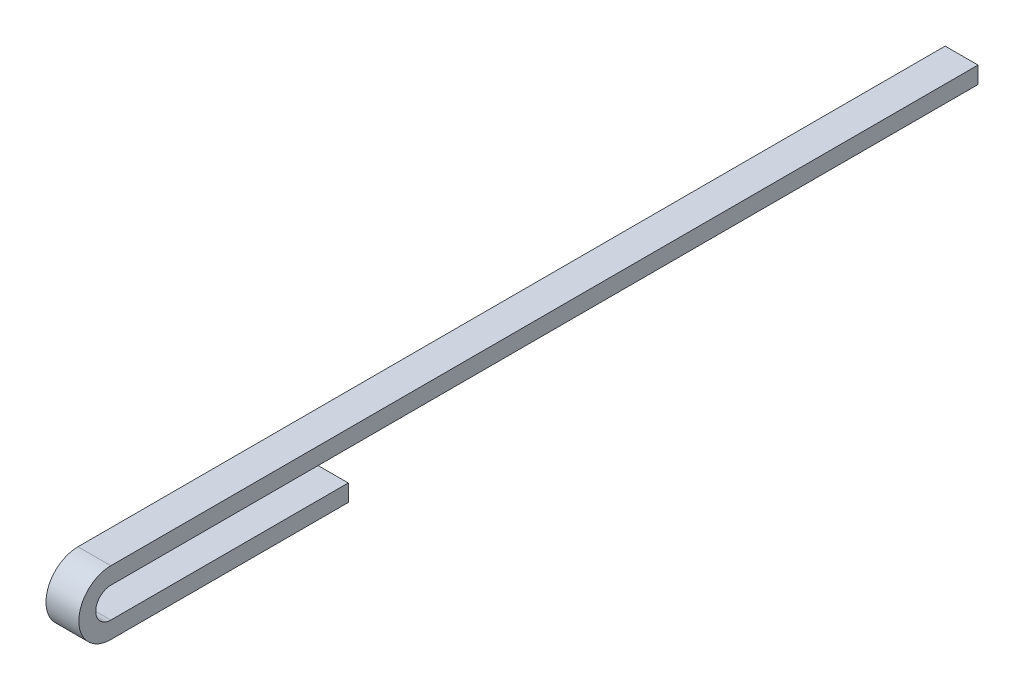
from build123d import *

# Parameters (mm, degrees)
EXTRUDE_1_DEPTH = 34


with BuildPart() as part:
    # 草图1 → 拉伸-薄壁1 (new, symmetric)
    with BuildSketch(Plane(origin=(-86.992315928, -141.229957863, -135.692636998), x_dir=(0, 0, -1), z_dir=(-1, 0, 0))):
        with BuildLine():
            Line((1100, 0), (-695.31480211, 0))
            ThreePointArc((-695.31480211, 0), (-761.535134985, 66.220332876), (-695.31480211, 132.440665751))
            Line((-695.31480211, 132.440665751), (-203.750159412, 132.440665751))
            Line((-203.750159412, 132.440665751), (-203.750159412, 97.440665751))
            Line((-203.750159412, 97.440665751), (-695.31480211, 97.440665751))
            ThreePointArc((-695.31480211, 97.440665751), (-726.535134985, 66.220332876), (-695.31480211, 35))
            Line((-695.31480211, 35), (1100, 35))
            Line((1100, 35), (1100, 0))
        make_face()
    extrude(amount=EXTRUDE_1_DEPTH, both=True)


solid = part.part
